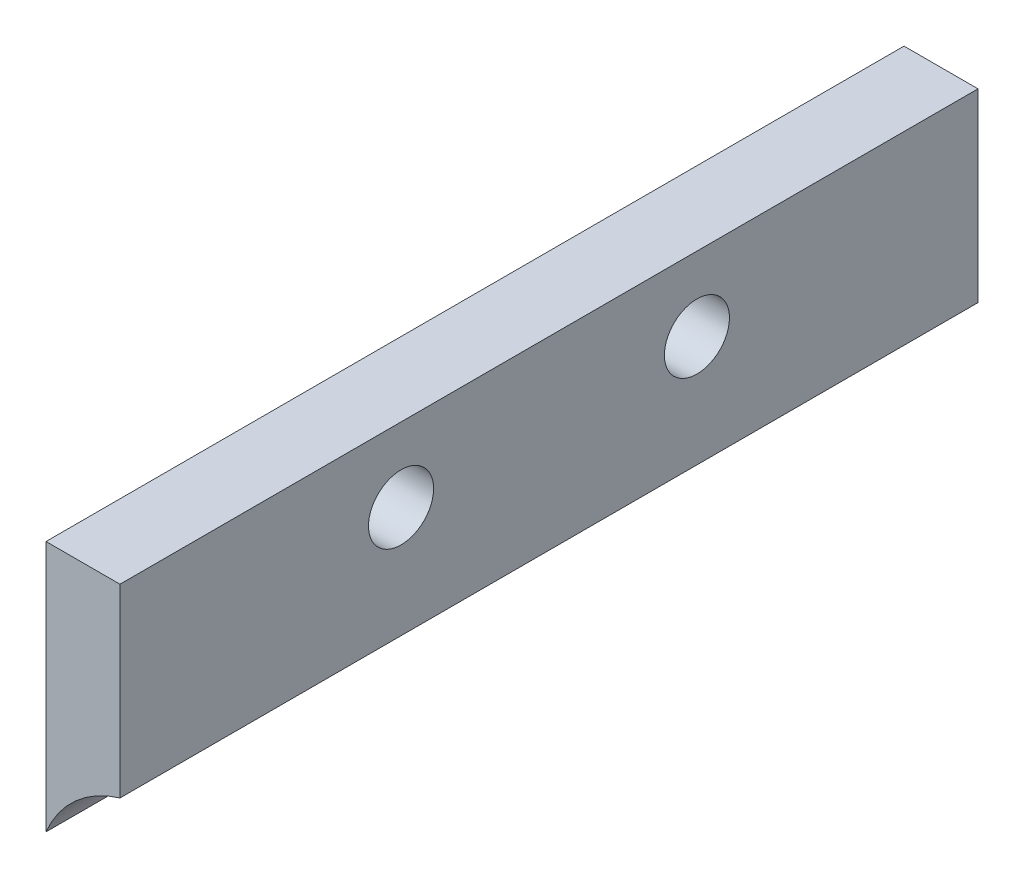
from build123d import *

# Parameters (mm, degrees)
EXTRUDE_1_DEPTH     = 58
SKETCH_2_R          = 2.2
CUT_EXTRUDE_1_DEPTH = 10


with BuildPart() as part:
    # 草图1 → 凸台-拉伸1 (new body)
    with BuildSketch(Plane.XY):
        with BuildLine():
            Line((-3.011664558, 4.541522048), (1.988335442, 4.541522048))
            Line((1.988335442, 4.541522048), (1.988335442, -7.975163179))
            ThreePointArc((1.988335442, -7.975163179), (-1.018873776, -9.651157386), (-3.011664558, -12.458477952))
            Line((-3.011664558, -12.458477952), (-3.011664558, 4.541522048))
        make_face()
    extrude(amount=EXTRUDE_1_DEPTH)

    # 草图2 → 切除-拉伸1 (cut)
    with BuildSketch(Plane(origin=(1.988335442, 0, 0), x_dir=(0, 0, -1), z_dir=(1, 0, 0))):
        with Locations(Location((-19, -0.458477952, 0), (0, 0, 90))):
            Circle(SKETCH_2_R)
        with Locations(Location((-39, -0.458477952, 0), (0, 0, 90))):
            Circle(SKETCH_2_R)
    extrude(amount=-CUT_EXTRUDE_1_DEPTH, mode=Mode.SUBTRACT)


solid = part.part
